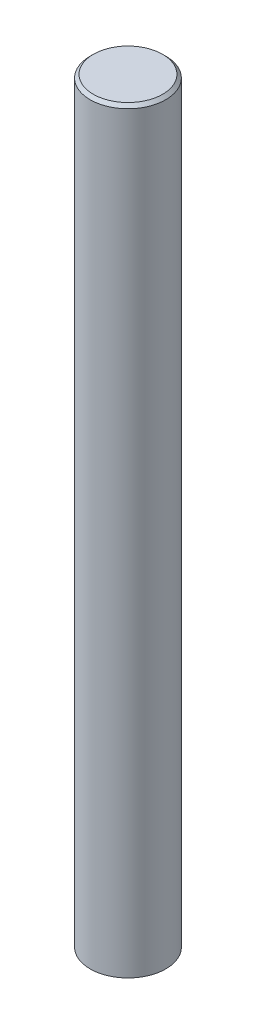
from build123d import *

# Parameters (mm, degrees)
SKETCH_1_R             = 6
EXTRUDE_1_DEPTH        = 120
HOLE_WIZARD_M4_1_D     = 3.3
HOLE_WIZARD_M4_1_DEPTH = 15.5
HOLE_WIZARD_M4_1_TIP   = 0.991420021
CHAMFER_1_SIZE         = 0.5


with BuildPart() as part:
    # 草图1 → 凸台-拉伸1 (new body)
    with BuildSketch(Plane(origin=(0, 0, 0), x_dir=(1, 0, 0), z_dir=(0, 1, 0))):
        with Locations(Location((0, 0, 0), (0, 0, 270))):
            Circle(SKETCH_1_R)
    extrude(amount=EXTRUDE_1_DEPTH)

    # M4 螺纹孔1
    with Locations(Plane(origin=(0, 0, 0), x_dir=(-1, 0, 0), z_dir=(0, -1, 0))):
        with Locations((0, 0)):
            Hole(HOLE_WIZARD_M4_1_D / 2, depth=HOLE_WIZARD_M4_1_DEPTH)
            with Locations((0, 0, -(HOLE_WIZARD_M4_1_DEPTH + HOLE_WIZARD_M4_1_TIP / 2))):  # 118° drill point
                Cone(0, HOLE_WIZARD_M4_1_D / 2, HOLE_WIZARD_M4_1_TIP, mode=Mode.SUBTRACT)

    # 倒角1
    chamfer_1_edges = [part.edges().sort_by_distance(p)[0] for p in [
        (0, 120, -6),
    ]]
    chamfer(chamfer_1_edges, length=CHAMFER_1_SIZE)


solid = part.part
